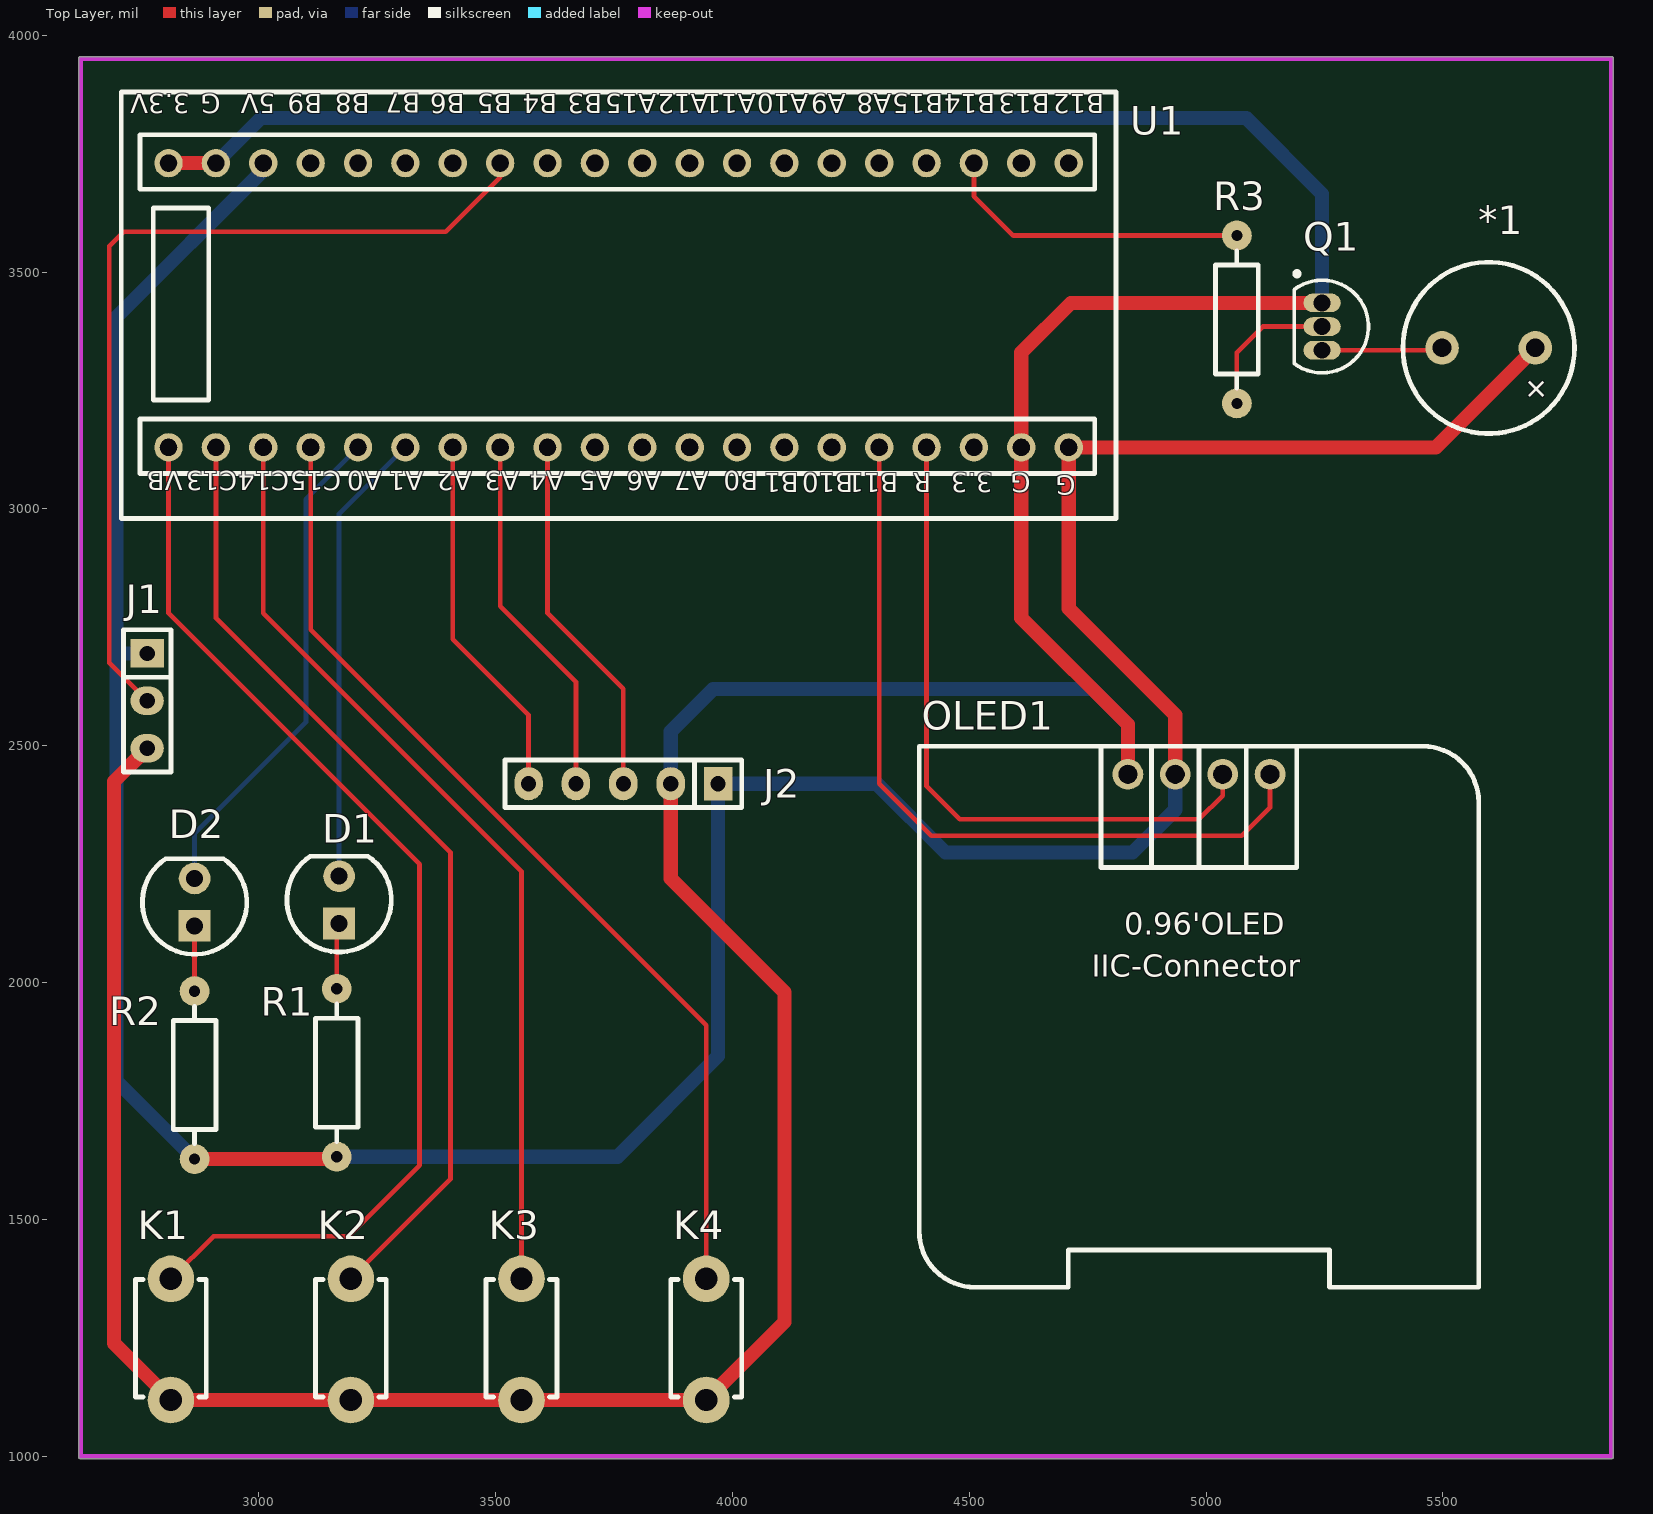
[diagram p0: Top Layer view]
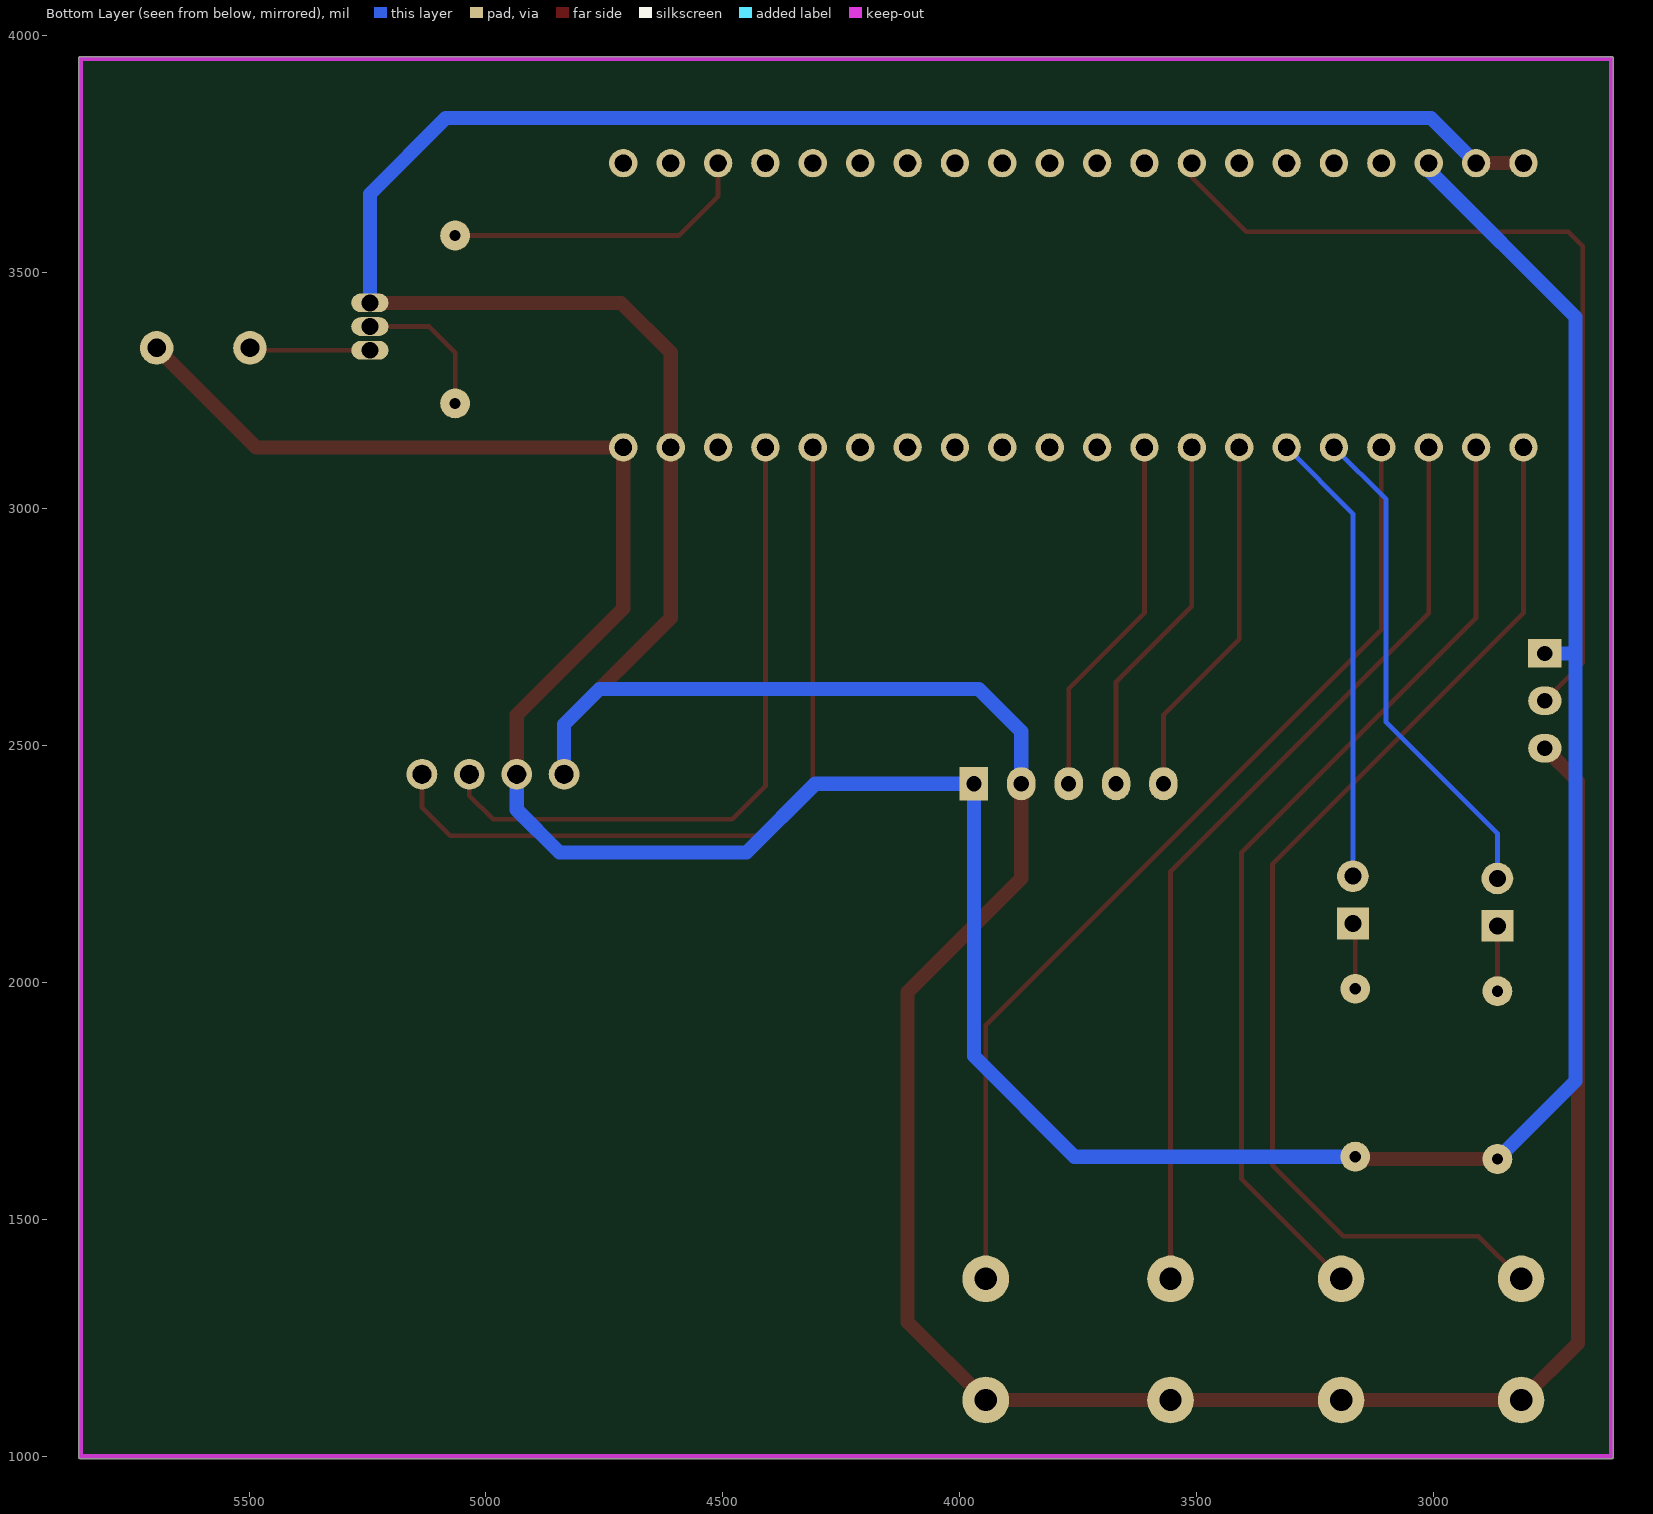
[diagram p1: Bottom Layer view, seen from below]
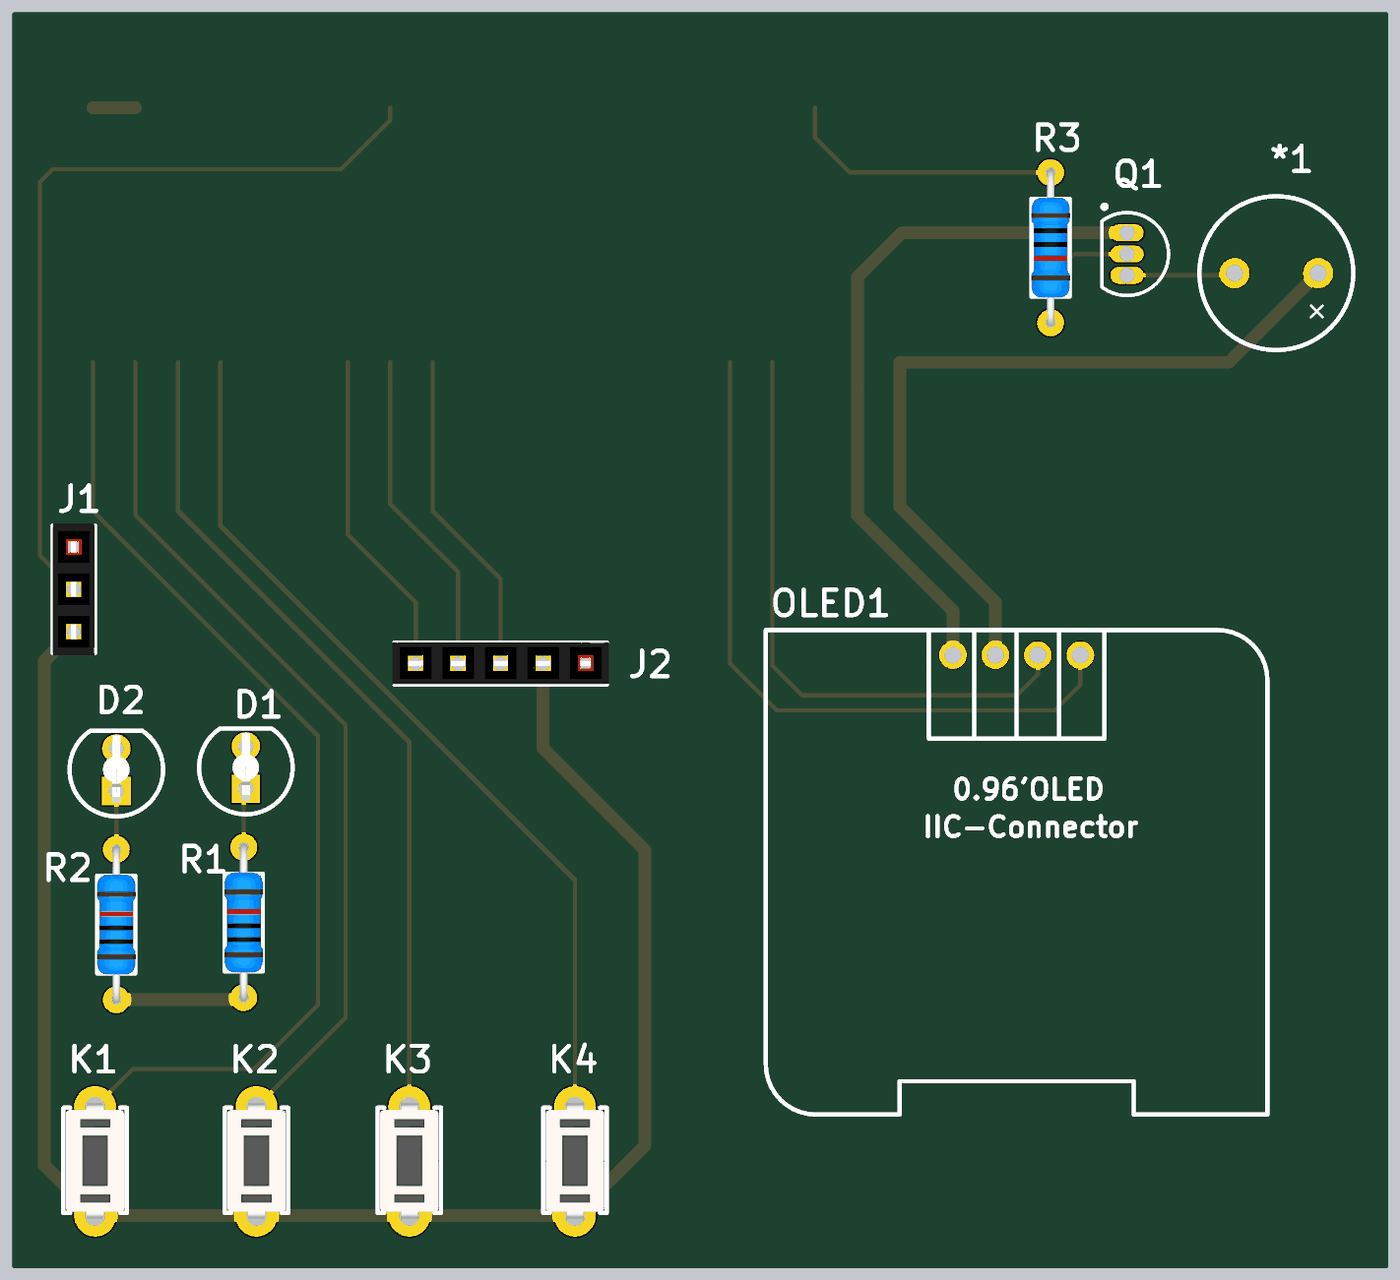
[diagram p2: 3D render of the assembled board from above, using the file's embedded part models]
# Altium PCB MISC80791.PcbDoc
Units mil, origin at the board's own origin, x right, y up, seen from the top; angles counter-clockwise.
Board outline 3240.03 x 2960.03 mil, 2 copper layers (Top Layer, Bottom Layer); 15 components, 21 nets, 75 pads, 0 vias.

## Layer stack, top to bottom (the 12.6 mil dielectric is the usual default, probably not edited)
Top Solder: solder mask 0.4, Solder Resist, Dk 3.5
Top Layer: signal copper 1.4
Dielectric 1: dielectric 12.6, FR-4, Dk 4.8
Bottom Layer: signal copper 1.4
Bottom Solder: solder mask 0.4, Solder Resist, Dk 3.5

## Board outline
2619.99,1000 ccw(c2625,1000) 2625,994.99 5855,994.99 ccw(c5855,1000) 5860.02,1000 5860.02,3950 ccw(c5855,3950) 5855,3955.01 2625,3955.01 ccw(c2625,3950) 2619.99,3950

## Design rules (kind name [scope] priority, off if disabled: settings)
Clearance [All] p1: gap=10
MinimumSolderMaskSliver [All] p1: minsoldermaskwidth=0
PolygonConnect [All] p1: connectstyle=Relief reliefconductorwidth=10 reliefentries=4 polygonreliefangle="90 Angle" airgapwidth=10
RoutingVias [All] p1: holewidth=28 width=50 viastyle="Through Hole" minholewidth=28 minwidth=50 maxholewidth=28 maxwidth=50
SilkToSilkClearance [All] p1: silktosilkclearance=0
SilkToSolderMaskClearance [IsPad] p1: minsilkscreentomaskgap=0 clearancetoexposedcopper=TRUE
SolderMaskExpansion [All] p1: expansion=4
Width [All] p1: maxlimit=30 minlimit=10 preferedwidth=10
27 further rules are at their usual default settings.

## Components (designator, comment, footprint, x,y, rotation, side; value= is the part's Value field where it differs from the comment)
*1 "Buzzer" BUZZER 5596.57,3340 r180 top
D1 "LED" "LED 5MM-W" 3170,2175 r90 top
D2 "LED" "LED 5MM-W" 2865,2170 r90 top
J1 "DHT11" Fe-HDR1X3/2.54-S 2765,2695 r0 top
J2 "DS1302" Fe-HDR1X5/2.54-S 3970,2420 r270 top
K1 "KEY" DIP-3X6X4.3 2815,1119.09 r90 top
K2 "KEY" DIP-3X6X4.3 3195,1119.09 r90 top
K3 "KEY" DIP-3X6X4.3 3555,1119.09 r90 top
K4 "KEY" DIP-3X6X4.3 3945,1119.09 r90 top
OLED1 "0.96OLED" 0.96OLED_4P 4985.05,1928.19 r0 top
Q1 "2N3904" TO-92A 5245,3385 r180 top
R1 "10K" "RS 1/4W" 3165,1810 r90 top
R2 "10K" "RS 1/4W" 2865,1805 r90 top
R3 "10K" "RS 1/4W" 5065,3400 r270 top
U1 "STM32F103C8T6 system board" STM32核心板 3536,4631.5 r90 top

## Footprints (in the part's own frame and the unit in brackets; to place one, negate y for a bottom-side part, rotate by r counter-clockwise, add the part's x,y. Pads: shape width x height; smd on the part's side, far side on the other; paste and mask are expansions set on the pad)
0.96OLED_4P [mm]
  round 1.65 hole 1 slot 1.005 at 0 deg paste+0 mask+0.051: 1(-3.811,12.997) 2(-1.271,13) 3(1.269,13) 4(3.809,13)
  silkscreen extent -15,-14.5 15,14.5
BUZZER [mm]
  round 1.8 hole 1 paste+0 mask+0.051: 1(-2.5,0) 2(2.5,0)
  silkscreen extent -4.6,-4.6 4.6,4.6
DIP-3X6X4.3 [mm]
  round 2.5 hole 1.2: 1(0,0) 3(6.5,0)
  silkscreen extent 0.16,-1.9 6.46,1.9, body extent -0.64,-1.75 7.19,1.75, height 4.31
Fe-HDR1X3/2.54-S [mil]
  rect 70x60 hole 32: 1(0,0)
  oval 70x60 hole 32: 2(0,-100) 3(0,-200)
  silkscreen extent -50,-250 50,50, body extent -50,-255 48,55, height 335
Fe-HDR1X5/2.54-S [mil]
  rect 70x60 hole 32: 1(0,0)
  oval 70x60 hole 32: 2(0,-100) 3(0,-200) 4(0,-300) 5(0,-400)
  silkscreen extent -50,-450 50,50, body extent -50,-455 48,55, height 126
"LED 5MM-W" [mm] "白色5mm直插LED"
  rect 1.7x1.7 hole 0.9: 1(-1.27,0)
  round 1.7 hole 0.9: 2(1.27,0)
  silkscreen extent -2.8,-2.8 2.33,2.8, body extent -2.85,-2.85 2.45,2.85, height 8.75
"RS 1/4W" [mm] "直插色环电阻，脚距9mm，直径2.3mm"
  round 1.6 hole 0.6: 1(-4.5,0) 2(4.5,0)
  silkscreen extent -3.68,-1.14 3.68,1.14, body extent -4.72,-1.16 4.73,1.16, height 2.32
STM32核心板 [mil]
  round 60 hole 36 slot 36.2 at 0 deg paste+0 mask+2: 1(-1501.5,726) 2(-1501.5,626) 3(-1501.5,526) 4(-1501.5,426) 5(-1501.5,326) 6(-1501.5,226) 7(-1501.5,126) 8(-1501.5,26) 9(-1501.5,-74) 10(-1501.5,-174) 11(-1501.5,-274) 12(-1501.5,-374) 13(-1501.5,-474) 14(-1501.5,-574) 15(-1501.5,-674) 16(-1501.5,-774) 17(-1501.5,-874) 18(-1501.5,-974) 19(-1501.5,-1074) 20(-1501.5,-1174) 21(-901.5,-1174) 22(-901.5,-1074) 23(-901.5,-974) 24(-901.5,-874) 25(-901.5,-774) 26(-901.5,-674) 27(-901.5,-574) 28(-901.5,-474) 29(-901.5,-374) 30(-901.5,-274) 31(-901.5,-174) 32(-901.5,-74) 33(-901.5,26) 34(-901.5,126) 35(-901.5,226) 36(-901.5,326) 37(-901.5,426) 38(-901.5,526) 39(-901.5,626) 40(-901.5,726)
  silkscreen extent -1652,-1274 -751,826
TO-92A [mm] "TO, Flat Index; 3 In-Line, Axial Leads; Body Dia. 4.5mm; Leads 0.51 x 0.48 mm (max)"
  oval 2x1 hole 0.9: 1(0,-1.27) 2(0,0) 3(0,1.27)
  silkscreen extent -2.48,-2.95 1.5,2.48, body extent -2.48,-2.5 1.5,2.5, height 6.86

## Part data
D1 D2: "Light-emitting diode"
J1: library part "Female HDR1X3"
J2: library part "Female HDR1X5"
OLED1: library part 0.96OLED_4P_MODULE_JX
Q1: "NPN General Purpose Amplifier"
R1 R2 R3: library part R-S, "Color-band resistor"
U1: library part STM32F103C8T6系统板

## Nets (pads, with @x,y where several pads share a name; then routed paths per layer and width w, separated by ;. In a path a pad name is that pad's centre, name@x,y a point inside that pad or via, vN(x,y) a via of type N, cw(c..) or ccw(c..) an arc to the next point about the centre after c; other vN are vias at no path point)
+5V: U1.18
ALARM: D2.2 U1.5 | length 1052.9
  Bottom Layer w10: D2.2 2865,2315 3100,2550 3100,3020 U1.5
BEEP: R3.1 U1.23 | length 659.3
  Top Layer w10: U1.23 4510,3660 4592.83,3577.17 R3.1
DHT11: J1.2 U1.33 | length 1908.2
  Top Layer w10: J1.2 2685,2675 2685,3555 2715,3585 3395,3585 3510,3700 U1.33
GND: J1.3 J2.2 K1.1 K2.1 K3.1 K4.1 OLED1.1 Q1.1 U1.19 U1.39 U1.40 | length 9734.1
  Top Layer w30: J1.3 2695,2425 2695,1239.09 K1.1 K2.1 K3.1 K4.1 4110,1284.09 4110,1980 3870,2220 J2.2 ; U1.40 U1.39 ; OLED1.1 4835,2545 4610,2770 U1.19 4610,3330 4715,3435 Q1.1
  Bottom Layer w30: U1.39 3005,3825 5085,3825 5245,3665 Q1.1 ; J2.2 3870,2530 3960,2620 4760,2620 4835,2545 OLED1.1
I/O: J2.4 U1.8 | length 776.3
  Top Layer w10: U1.8 3510,2795 3670,2635 J2.4
KEY1: K1.3 U1.1 | length 2358.9
  Top Layer w10: U1.1 2810,2780 3340,2250 3340,1615 3190,1465 2905,1465 K1.3
KEY2: K2.3 U1.2 | length 2047
  Top Layer w10: U1.2 2910,2770 3405,2275 3405,1585 K2.3
KEY3: K3.3 U1.3 | length 1980.7
  Top Layer w10: U1.3 3010,2780 3555,2235 K3.3
KEY4: K4.3 U1.4 | length 2100.9
  Top Layer w10: U1.4 3110,2745 3945,1910 K4.3
LIMT: D1.2 U1.6 | length 963
  Bottom Layer w10: D1.2 3170,2990 U1.6
Net*1_2: *1.2 Q1.3 | length 255.2
  Top Layer w10: Q1.3 5493.15,3335 *1.2
NetD1_1: D1.1 R1.2 | length 139.9
  Top Layer w10: R1.2 3165,2120 D1.1
NetD2_1: D2.1 R2.2 | length 137.8
  Top Layer w10: R2.2 D2.1
NetQ1_2: Q1.2 R3.2 | length 309.9
  Top Layer w10: R3.2 5065,3330 5120,3385 Q1.2
NetSW1_2: 
RST: J2.5 U1.7 | length 776.3
  Top Layer w10: U1.7 3410,2725 3570,2565 J2.5
SCL: OLED1.3 U1.17 | length 1434.7
  Top Layer w10: U1.17 4410,2415 4480,2345 4985,2345 5035,2395 OLED1.3
SCLK: J2.3 U1.9 | length 776.3
  Top Layer w10: U1.9 3610,2780 3770,2620 J2.3
SDA: OLED1.4 U1.16 | length 1675.4
  Top Layer w10: U1.16 4310,2420 4420,2310 5075,2310 5135,2370 OLED1.4
VCC: *1.1 J1.1 J2.1 OLED1.2 R1.1 R2.1 U1.20 U1.38 | length 7126.4
  Top Layer w30: R2.1 3160,1627.83 R1.1 ; OLED1.2 4935,2565 4710,2790 U1.20 5485,3130 *1.1
  Bottom Layer w30: J1.1 2700,2695 ; R2.1 2700,1792.83 2700,2695 ; U1.38 3010,3715 2700,3405 2700,2695 ; R1.1 3757.83,1632.83 3970,1845 J2.1 4305,2420 4450,2275 4845,2275 4935,2365 OLED1.2
pads on no net: U1.10 U1.11 U1.12 U1.13 U1.14 U1.15 U1.21 U1.22 U1.24 U1.25 U1.26 U1.27 U1.28 U1.29 U1.30 U1.31 U1.32 U1.34 U1.35 U1.36 U1.37

## Keep-outs
Keep-Out Layer:
  lines w10: 2625,3885 2625,3950 5855,3950 5855,1000 2625,1000 2625,3900